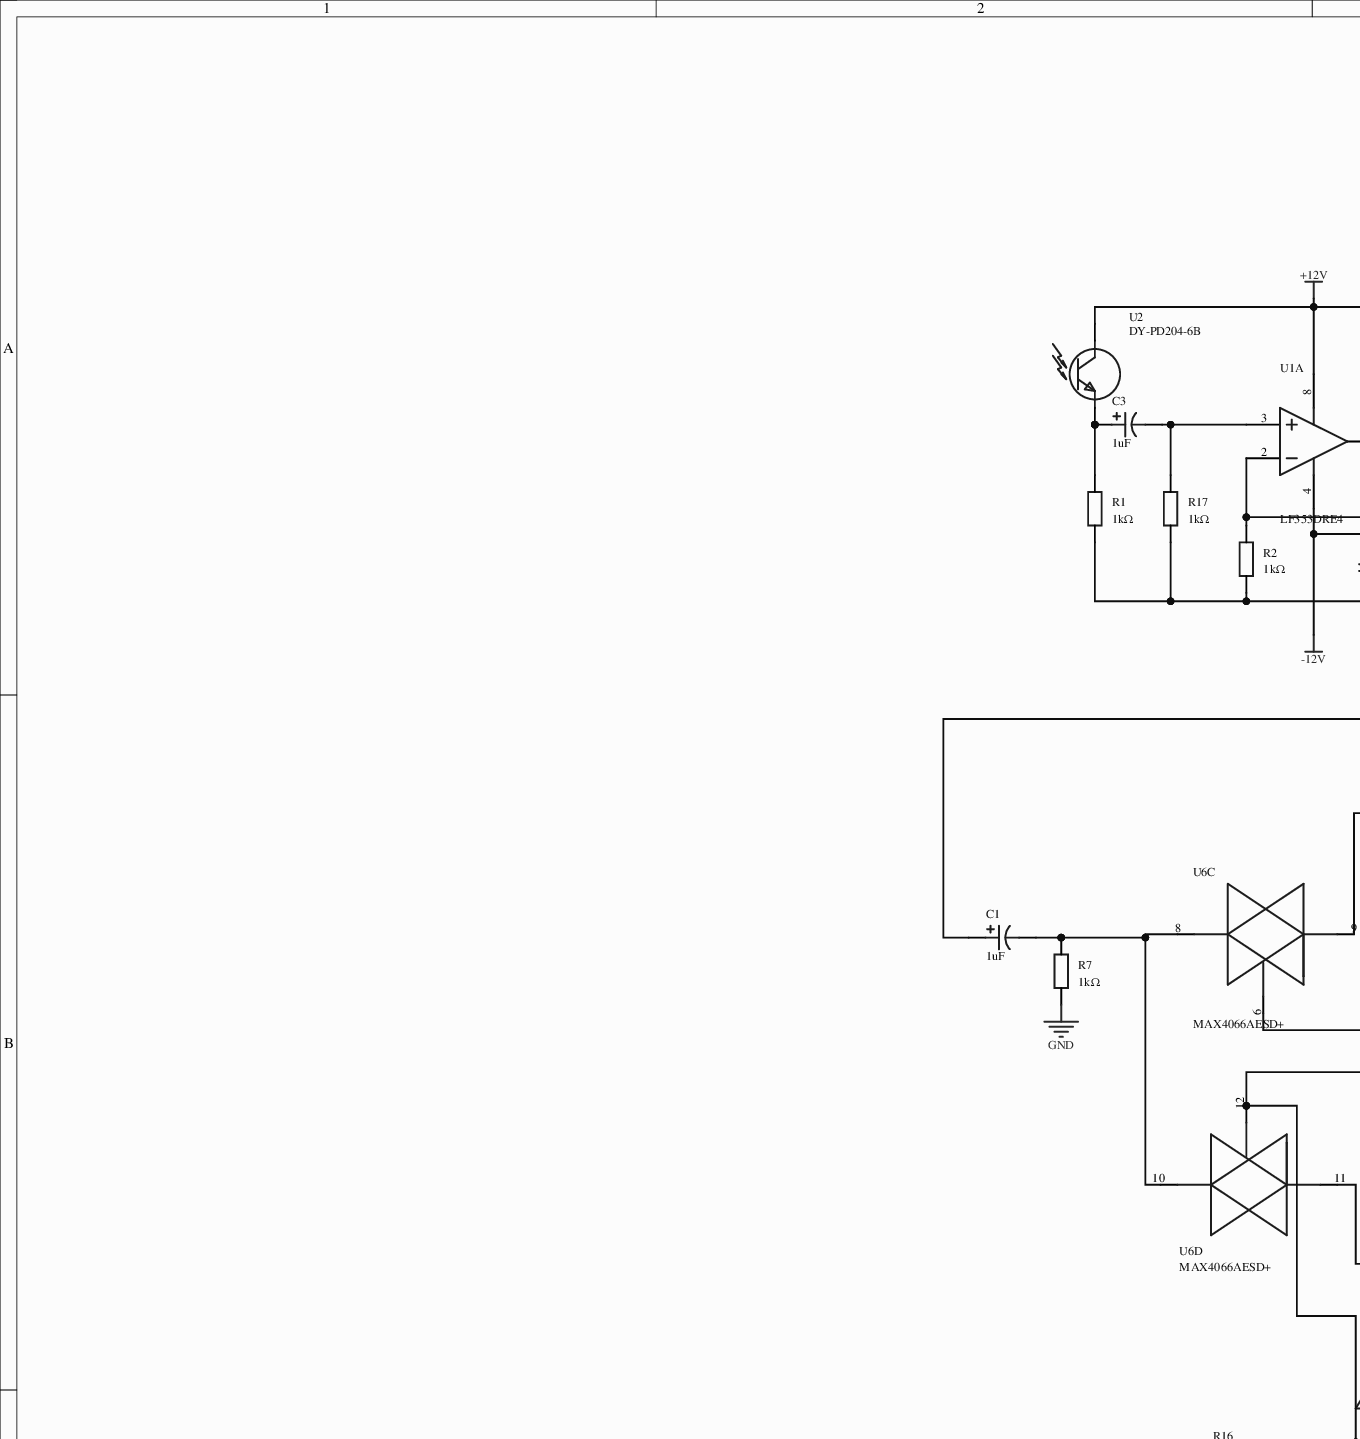
[diagram p0: MISC51811-3.schdoc, top left]
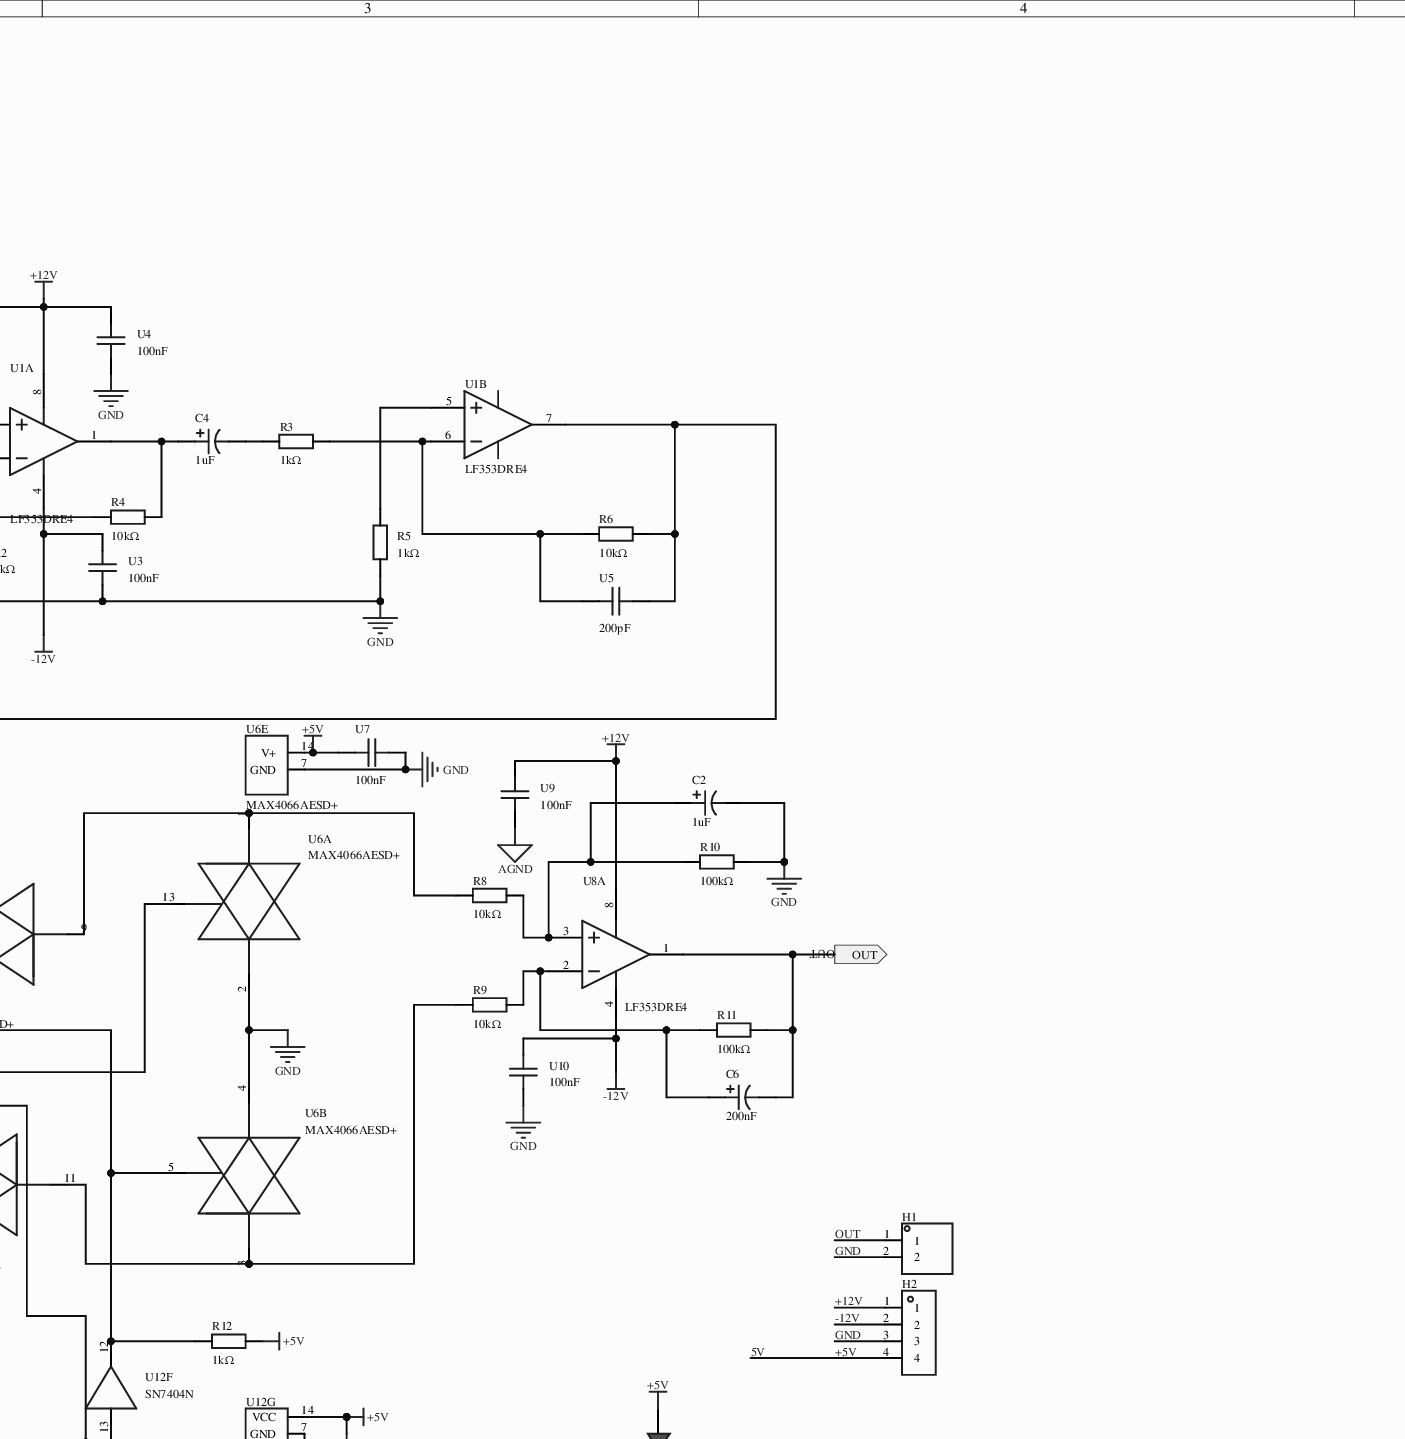
[diagram p1: MISC51811-3.schdoc, top middle]
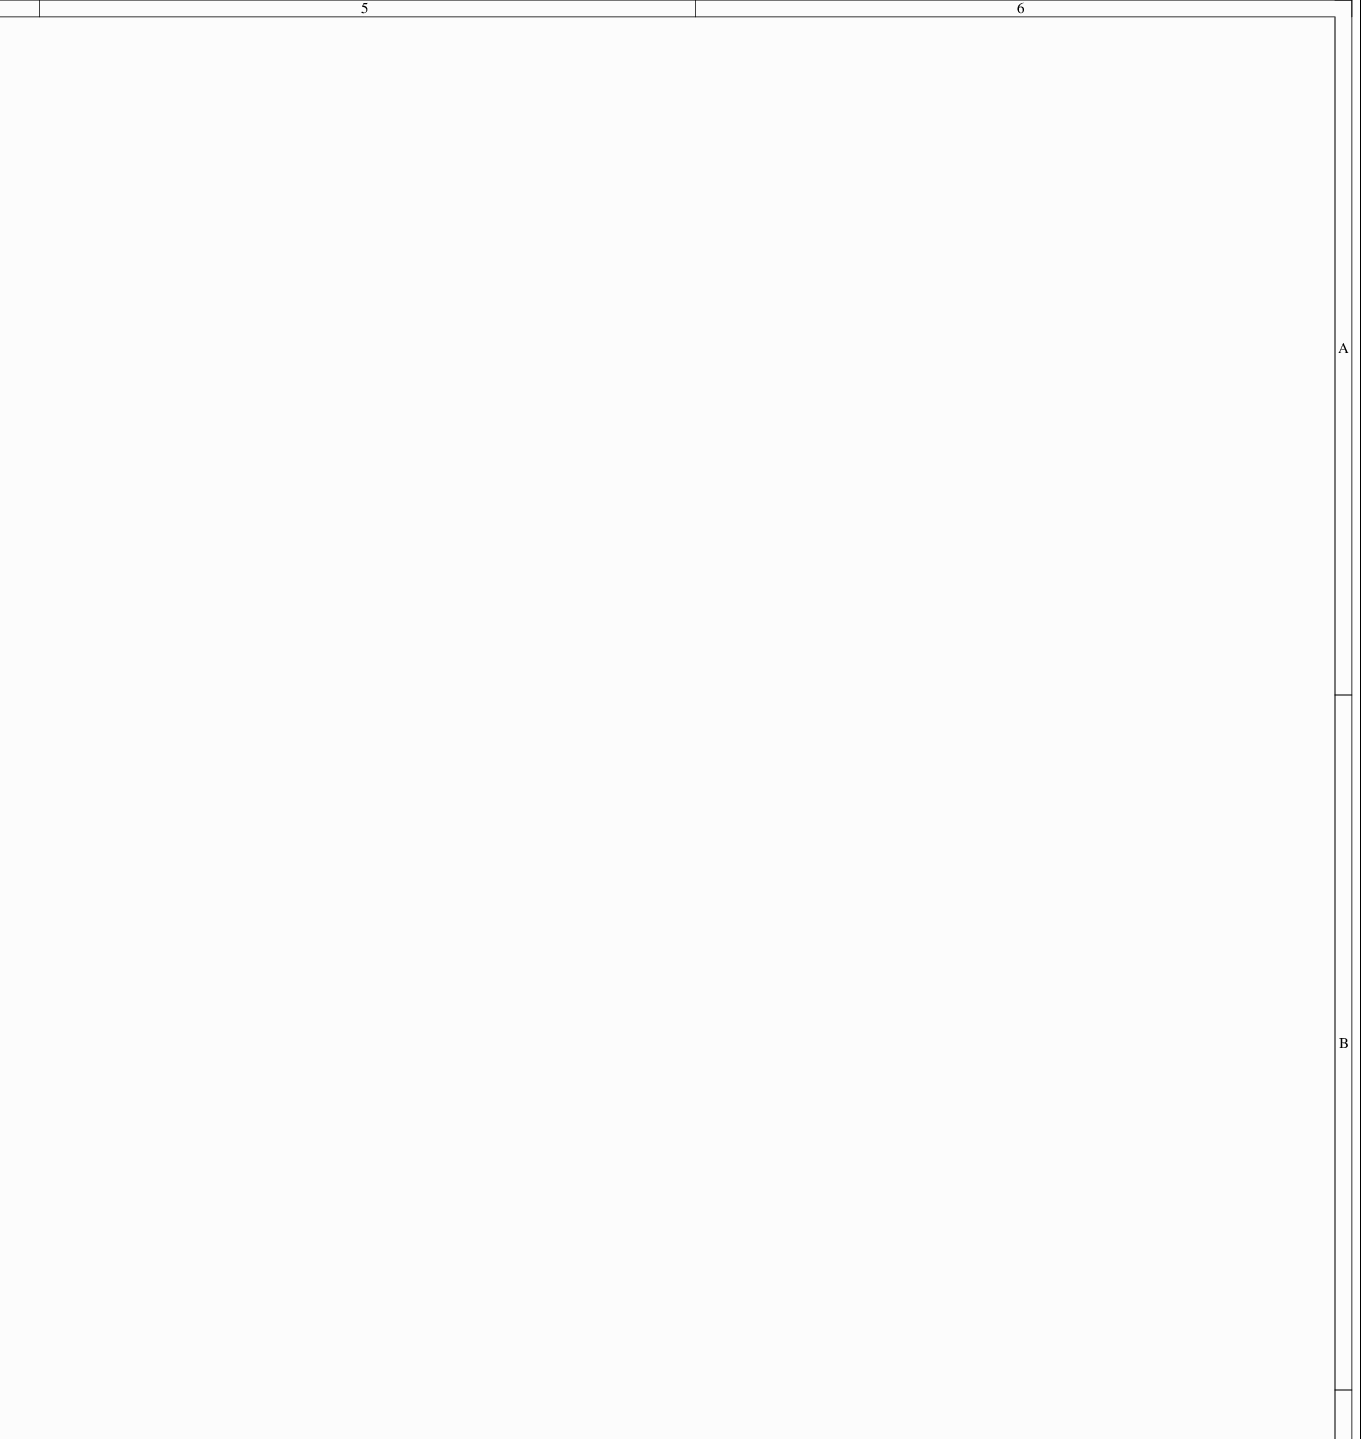
[diagram p2: MISC51811-3.schdoc, top right]
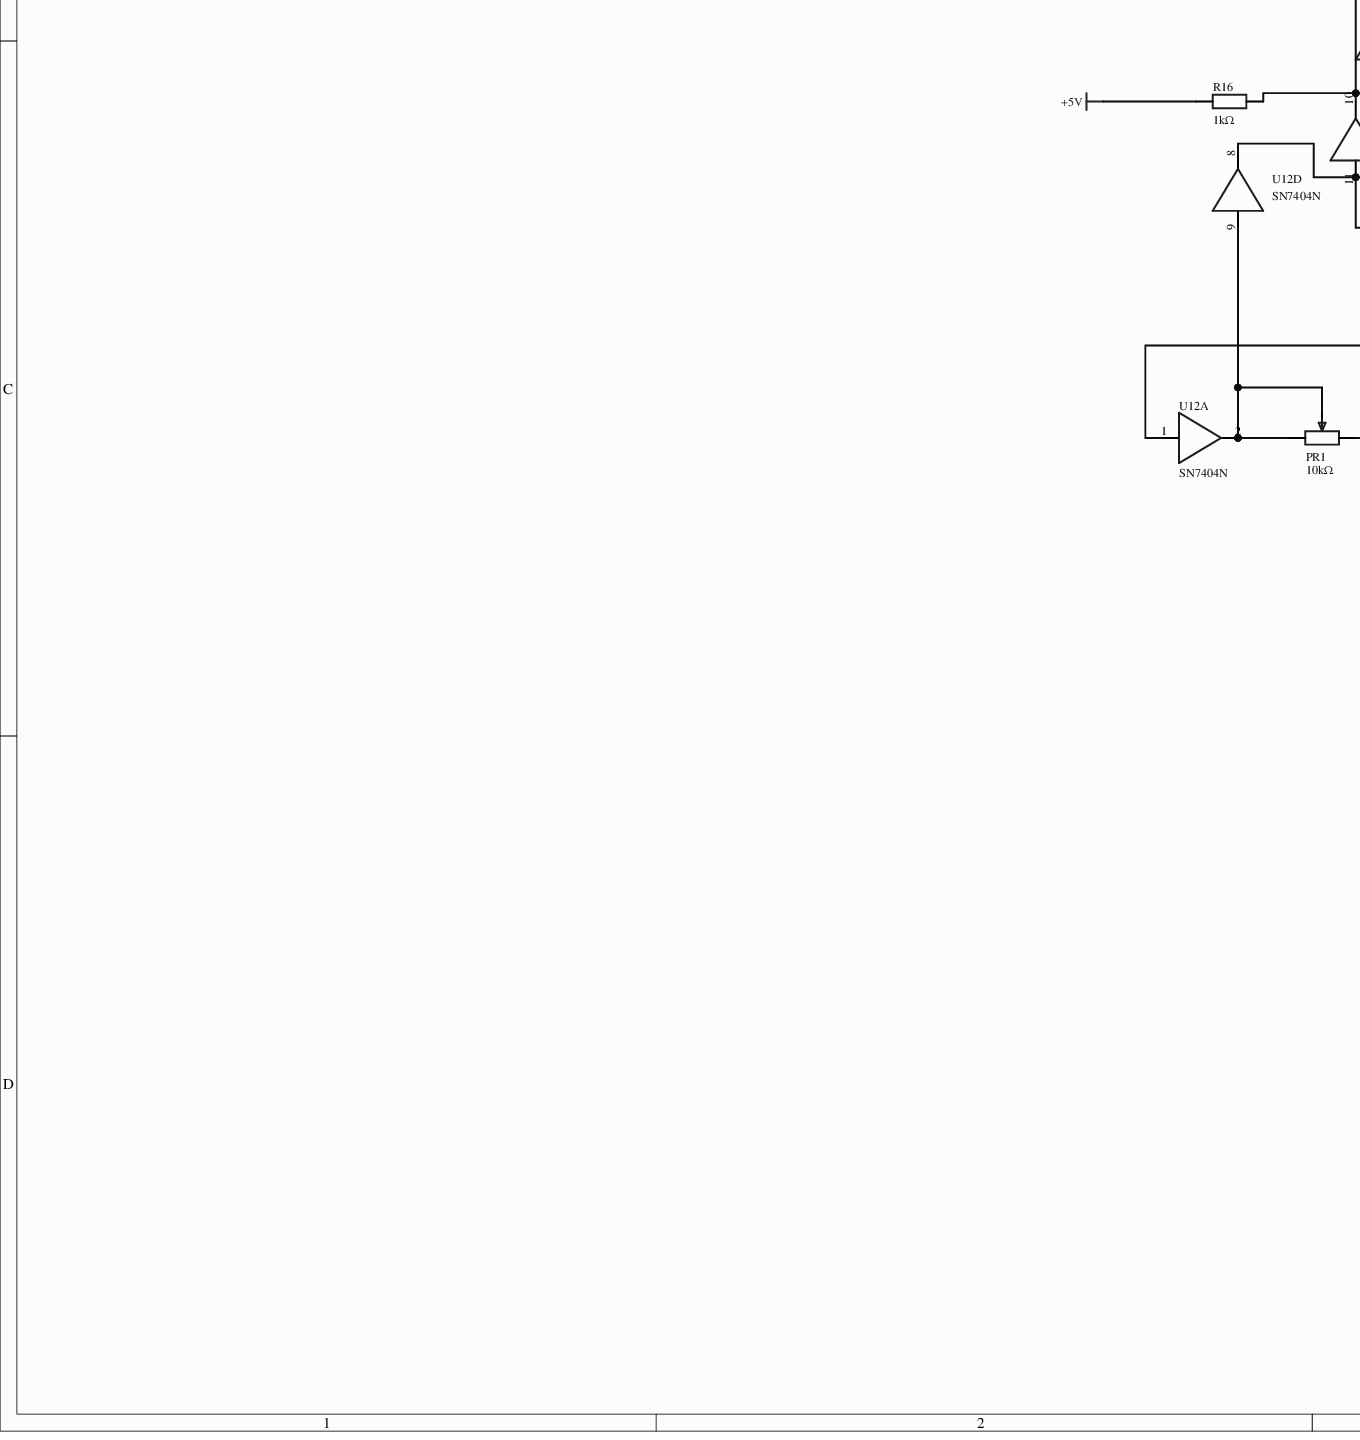
[diagram p3: MISC51811-3.schdoc, bottom left]
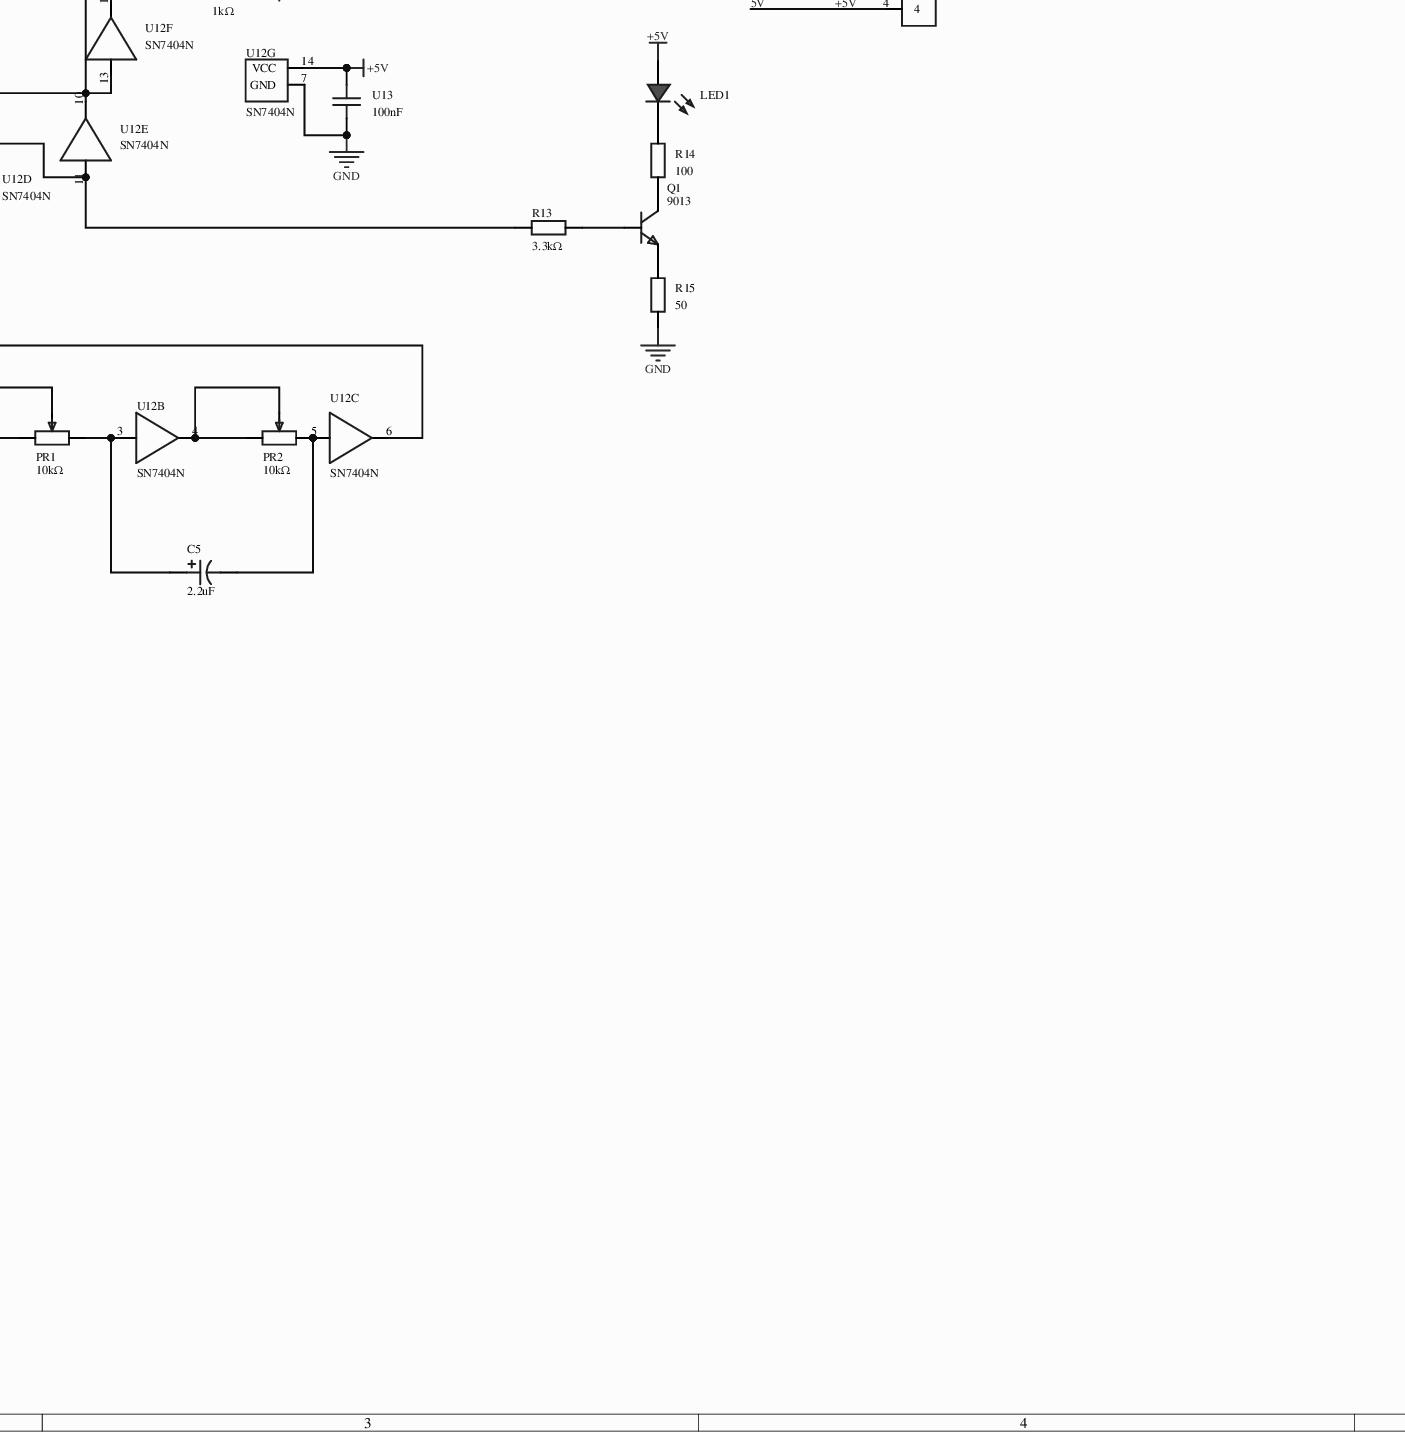
[diagram p4: MISC51811-3.schdoc, bottom middle]
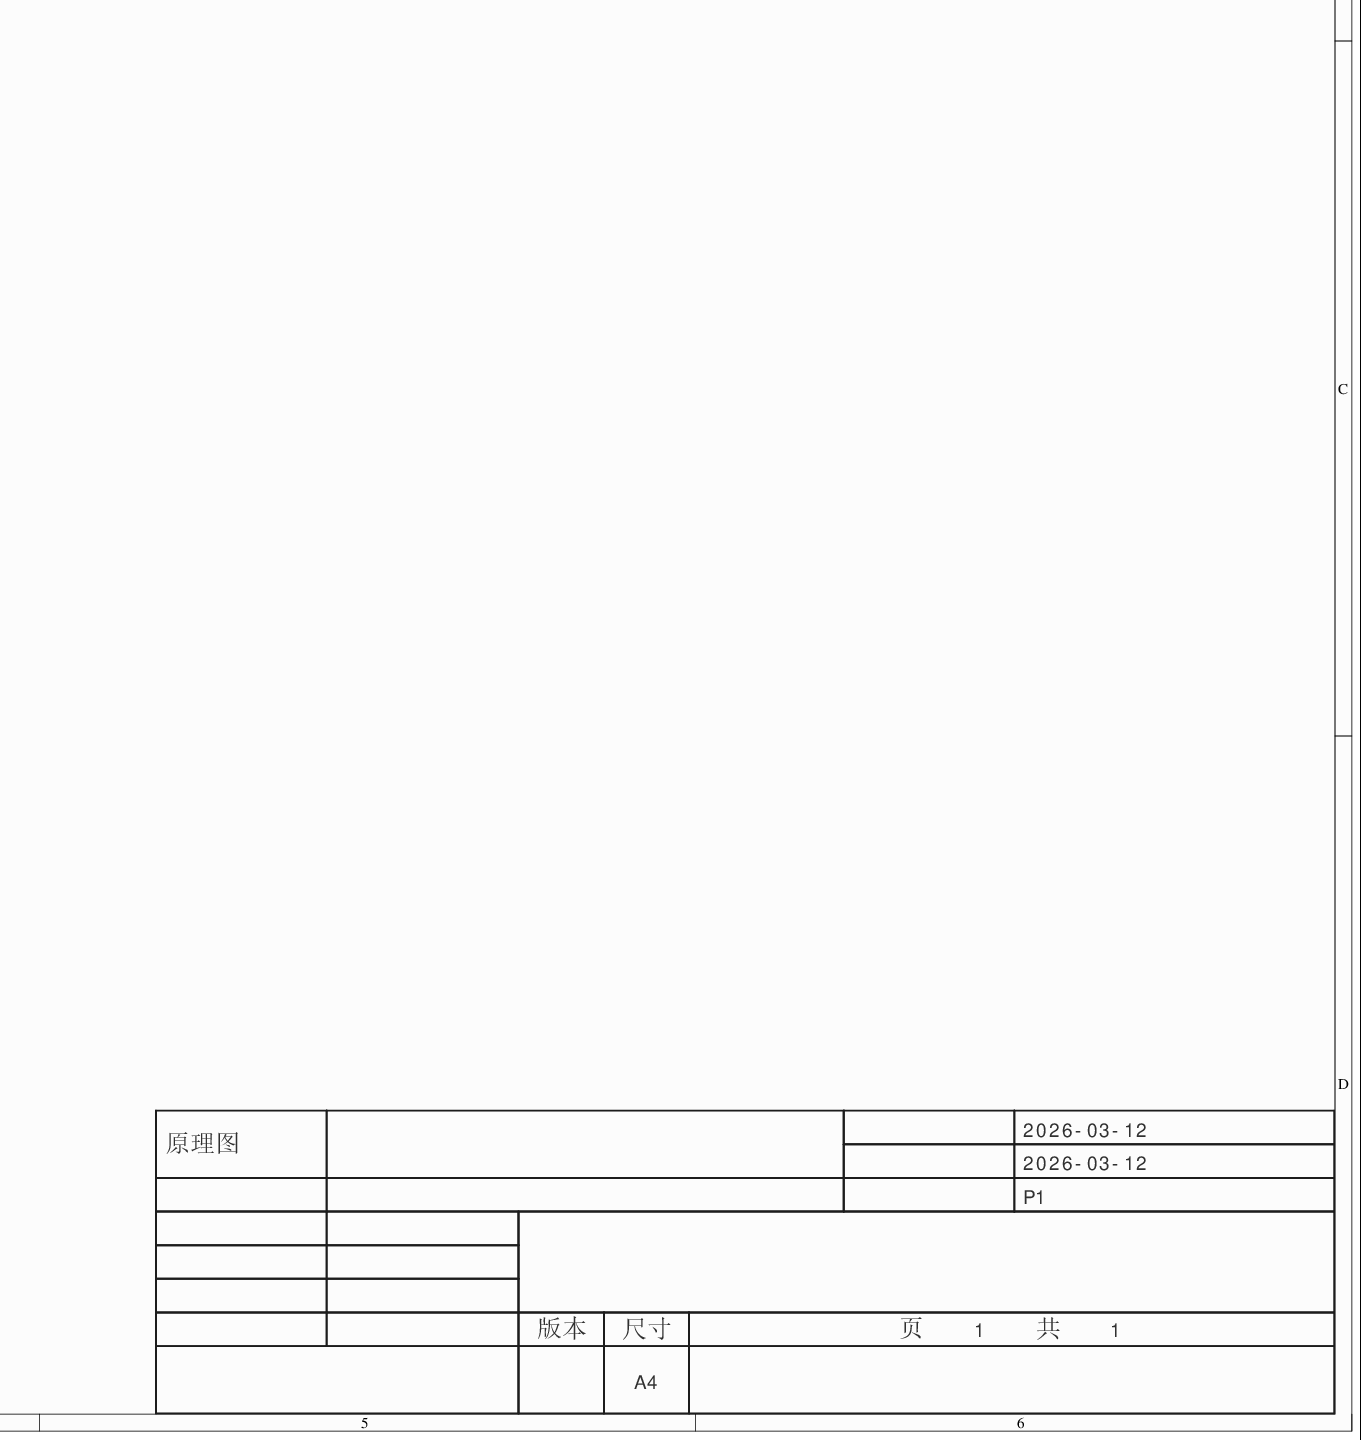
[diagram p5: MISC51811-3.schdoc, bottom right]
# Altium project MISC51811-2.PrjPcb
1 sheet, 41 parts. Net scope: flat (ports and power ports of the same name join across sheets).
Board file: MISC51811.pcbdoc

## Sheet MISC51811-3.schdoc
size 594 x 419 mm; Version: V1.0; @Project Name: MISC51811; @Update Date: 2026-03-12; @Create Date: 2026-03-12; @Board Name: MISC51811; @Create Time: 18:01:41; @Page Count: 1; @Page No: 1; @Schematic Name: MISC51811; @Update Time: 18:01:41; Size: A4

### Parts
C1  1uF  [CAP-TH_BD6.3-P2.50-D0.5-FD]
C2  1uF  [CAP-TH_BD6.3-P2.50-D0.5-FD]
C3  1uF  [CAP-TH_BD6.3-P2.50-D0.5-FD]
C4  1uF  [CAP-TH_BD6.3-P2.50-D0.5-FD]
C5  2.2uF  [CAP-TH_BD8.0-P3.50-D0.5-FD]
C6  200nF  [CAP-TH_BD6.3-P2.50-D0.5-FD]
H1  (no value)  [HDR-TH_2P-P2.54-V-M-1]
H2  (no value)  [HDR-TH_4P-P2.54-V-M]
LED1  (no value)  [LED_TH-3mm]
PR1  10kΩ  [R_3296]
PR2  10kΩ  [R_3296]
Q1  9013  [TO-92-3_L4.8-W3.7-P2.54-R]
R1  1kΩ  [Res_1/8W]
R2  1kΩ  [Res_1/8W]
R3  1kΩ  [Res_1/8W]
R4  10kΩ  [Res_1/8W]
R5  1kΩ  [Res_1/8W]
R6  10kΩ  [Res_1/8W]
R7  1kΩ  [Res_1/8W]
R8  10kΩ  [Res_1/8W]
R9  10kΩ  [Res_1/8W]
R10  100kΩ  [Res_1/8W]
R11  100kΩ  [Res_1/8W]
R12  1kΩ  [Res_1/8W]
R13  3.3kΩ  [Res_1/8W]
R14  100  [Res_1/8W]
R15  50  [Res_1/8W]
R16  1kΩ  [Res_1/8W]
R17  1kΩ  [Res_1/8W]
U1  LF353DRE4  [SOIC-8_L5.0-W4.0-P1.27-LS6.1-BL]  (parts A,B of 2)
U2  DY-PD204-6B  [LED-TH_BD3.0-P2.54-FD]
U3  100nF  [CAP-TH_L5.0-W2.5-P5.00-D1.0]
U4  100nF  [CAP-TH_L5.0-W2.5-P5.00-D1.0]
U5  200pF  [CAP-TH_L4.9-W3.7-P5.08-D0.5]
U6  MAX4066AESD+  [SOIC-14_L8.7-W3.9-P1.27-LS6.0-BL]  (parts A,B,C,D,E of 5)
U7  100nF  [CAP-TH_L5.0-W2.5-P5.00-D1.0]
U8  LF353DRE4  [SOIC-8_L5.0-W4.0-P1.27-LS6.1-BL]  (part A of 2)
U9  100nF  [CAP-TH_L5.0-W2.5-P5.00-D1.0]
U10  100nF  [CAP-TH_L5.0-W2.5-P5.00-D1.0]
U12  SN7404N  [PDIP-14_L19.3-W6.4-P2.54-LS7.9-BL-1]  (parts A,B,C,D,E,F,G of 8)
U13  100nF  [CAP-TH_L5.0-W2.5-P5.00-D1.0]

### Ports
OUT (out)

### Nets
+5V: H2.4 LED1.1(C) R12.1 R16.1 U6.14(V+) U7.1 U12.14(VCC) U13.2  [also labelled 5V]
+12V: H2.1 U1.8(VCC+) U2.2(C) U4.1 U8.8(VCC+) U9.2
-12V: H2.2 U1.4(VCC-) U3.1 U8.4(VCC-) U10.2
AGND: U9.1
GND: C2.2 H1.2 H2.3 R1.1 R2.1 R5.2 R7.1 R10.2 R15.1 R17.1 U3.2 U4.2 U6.2(COM1) U6.4(COM1) U6.7(GND) U7.2 U10.1 U12.7(GND) U13.1
OUT: C6.2 H1.1 R11.2 U8.1(1OUT) ; port OUT
NetC1_1: C1.1 R6.2 U1.7(2OUT) U5.2
NetC1_2: C1.2 R7.2 U6.8(COM1) U6.10(COM1)
NetC2_1: C2.1 R8.2 R10.1 U8.3(1IN-)
NetC3_1: C3.1 R1.2 U2.1(E)
NetC3_2: C3.2 R17.2 U1.3(1IN-)
NetC4_1: C4.1 R4.2 U1.1(1OUT)
NetC4_2: C4.2 R3.2
NetC5_1: C5.1 PR1.1 U12.3(1Y)
NetC5_2: C5.2 PR2.1 U12.5(1Y)
NetC6_1: C6.1 R9.2 R11.1 U8.2(1IN+)
NetLED1_2: LED1.2(A) R14.2
NetPR1_2: PR1.2 PR1.3 U12.2(1A) U12.9(1Y)
NetPR2_2: PR2.2 PR2.3 U12.4(1A)
NetQ1_1: Q1.1(C) R14.1
NetQ1_2: Q1.2(B) R13.2
NetQ1_3: Q1.3(E) R15.2
NetR2_2: R2.2 R4.1 U1.2(1IN+)
NetR3_1: R3.1 R6.1 U1.6(2IN-) U5.1
NetR5_1: R5.1 U1.5(2IN+)
NetR8_1: R8.1 U6.1(NO1) U6.9(NO1)
NetR9_1: R9.1 U6.3(NO1) U6.11(NO1)
NetR12_2: R12.2 U6.5(IN1) U6.6(IN1) U12.12(1A)
NetR13_1: R13.1 U12.8(1A) U12.11(1Y)
NetR16_2: R16.2 U6.12(IN1) U6.13(IN1) U12.10(1A) U12.13(1Y)
NetU12_1: U12.1(1Y) U12.6(1A)

### Notes on the sheet
- 2026-03-12
- 原理图
- P1
- 版本
- 尺寸
- A4
- 页    1    共    1

### Library data of the parts
C1-C4 = 1uF450V6.3x12KM: 容值:1uF;精度:±20%;额定电压:450V;纹波电流:545mA@120Hz;等效串联电阻(ESR):11Ω;; Manufacturer: Econd(米朗电子); AddInBom: yes; ModelId: 983aa343eddc42b59ebb10541a88166e0819f05c4eef4c71ace90d822a990e87; ModelTransform: 247.99486,248.229,0,90,0,0,0,0,-196.85; Tolerance: ±20%; Voltage Rating: 450V; Equivalent Series Resistance(ESR): 11Ω; Pin Spacing: 2.5mm; Lifetime: 2000hrs@105℃; Symbol: 1UF450V6.3X12KM; Device: 1uF450V6.3x12KM; LCSC Part Name: 1uF ±20% 450V; SupplierPart: C49304904; ManufacturerPart: 1uF450V6.3x12KM; Supplier Footprint: 插件,D6.3xL12mm; JLCPCB Part Class: Extended Part; Datasheet: https://item.szlcsc.com/datasheet/1uF450V6.3x12KM/51766732.html; Supplier: LCSC; ConvertToPcb: yes; FootprintName: CAP-TH_BD6.3-P2.50-D0.5-FD; ModelName: CAP-TH_BD6.3-P2.50-D0.5-FD; Value: 1uF; Ripple Current: 545mA@120Hz; Diameter: 6.3mm; Height - Seated (Max): 12mm; Operating Temperature: -25℃~+105℃
C5 = 2.2uF450V8x12KM: 容值:2.2uF;精度:±20%;额定电压:450V;纹波电流:35mA@120HZ;等效串联电阻(ESR):11Ω;; Manufacturer: Econd(米朗电子); AddInBom: yes; ModelId: 627d55c9ca1c4b51a61bba7c83a7ae6f0819f05c4eef4c71ace90d822a990e87; ModelTransform: 314.96,315.3537,0,90,0,0,0,0,-196.85; Tolerance: ±20%; Voltage Rating: 450V; Equivalent Series Resistance(ESR): 11Ω; Pin Spacing: 3.5mm; Lifetime: 2000hrs@105℃; Symbol: 2.2UF450V8X12KM; Device: 2.2uF450V8x12KM; LCSC Part Name: 2.2uF ±20% 450V; SupplierPart: C49304892; ManufacturerPart: 2.2uF450V8x12KM; Supplier Footprint: 插件,D8xL12mm; JLCPCB Part Class: Extended Part; Datasheet: https://item.szlcsc.com/datasheet/2.2uF450V8x12KM/51766720.html; Supplier: LCSC; ConvertToPcb: yes; FootprintName: CAP-TH_BD8.0-P3.50-D0.5-FD; ModelName: CAP-TH_BD8.0-P3.50-D0.5-FD; Value: 2.2uF; Ripple Current: 35mA@120HZ; Diameter: 8mm; Height - Seated (Max): 12mm; Operating Temperature: -25℃~+105℃
C6 = 1uF450V6.3x12KM: 容值:1uF;精度:±20%;额定电压:450V;纹波电流:545mA@120Hz;等效串联电阻(ESR):11Ω;; Manufacturer: Econd(米朗电子); 3D Model: 983aa343eddc42b59ebb10541a88166e0819f05c4eef4c71ace90d822a990e87; 3D Model Transform: 247.99486,248.229,0,90,0,0,0,0,-196.85; Tolerance: ±20%; Voltage Rating: 450V; Equivalent Series Resistance(ESR): 11Ω; Pin Spacing: 2.5mm; Lifetime: 2000hrs@105℃; AddInBom: yes; Symbol: 1UF450V6.3X12KM; Device: 1uF450V6.3x12KM; LCSC Part Name: 1uF ±20% 450V; Manufacturer Part: 1uF450V6.3x12KM; Supplier Footprint: 插件,D6.3xL12mm; JLCPCB Part Class: Extended Part; Datasheet: https://item.szlcsc.com/datasheet/1uF450V6.3x12KM/51766732.html; Supplier: LCSC; Value: 200nF; Ripple Current: 545mA@120Hz; Diameter: 6.3mm; Height - Seated (Max): 12mm; Operating Temperature: -25℃~+105℃; ConvertToPcb: yes; FootprintName: CAP-TH_BD6.3-P2.50-D0.5-FD; ModelName: CAP-TH_BD6.3-P2.50-D0.5-FD
H1 = HDR-M_2.54_1x2P: Symbol: 210S-1*2P L=11.6MMGold-plated black; ConvertToPcb: yes; ModelId: 79b2e9f2d70a4d68a1b7098f27c6d4c50819f05c4eef4c71ace90d822a990e87; ModelName: HDR-M-2.54_1x2; ModelTransform: 200,100,0,0,0,0,0,0,-118.11; Device: HDR-M_2.54_1x2P; AddInBom: yes; SupplierPart: C124375; Supplier Footprint: 插件; FootprintName: HDR-TH_2P-P2.54-V-M-1
H2 = HDR-M_2.54_1x4P: Symbol: PZ254V-11-04P; ConvertToPcb: yes; ModelId: 112f4d05e8d64e99ab9a333894bea4f90819f05c4eef4c71ace90d822a990e87; ModelName: HDR-TH_4P-P2.54-M-LI-1X4P; ModelTransform: 399.999,104.7242,0,0,0,0,0,0,-118.11; Device: HDR-M_2.54_1x4P; AddInBom: yes; SupplierPart: C492403; Supplier Footprint: 插件; FootprintName: HDR-TH_4P-P2.54-V-M
LED1 = LED_TH-R_3mm: ConvertToPcb: yes; ModelId: a497c992633541038a38947cdc58012f0819f05c4eef4c71ace90d822a990e87; ModelName: LED-TH-3mm_R; ModelTransform: 141.274,153.327,0,0,0,0,-5.984,0,-137.795; Symbol: LED_TH-R; Device: LED_TH-R_3mm; AddInBom: yes; FootprintName: LED_TH-3mm; Supplier Footprint: 插件
PR1 PR2 = R_3296: ConvertToPcb: yes; ModelId: b182808559bb43bda9e7de64b64134cb0819f05c4eef4c71ace90d822a990e87; ModelName: 3296W; ModelTransform: 373.98,188.96,590.49,180,0,0,0,0,-140; Symbol: R_3296; Device: R_3296; AddInBom: yes; Supplier Footprint: 直插; FootprintName: R_3296; Value: 10kΩ
Q1 = 9013: 晶体管类型:NPN;集电极电流(Ic):500mA;集射极击穿电压(Vceo):20V;耗散功率(Pd):625mW;直流电流增益(hFE):276@50mA,1.0V;; Manufacturer: BLUE ROCKET(蓝箭); AddInBom: yes; ModelId: 0fb83455cf6d479b95862acdd73b6eef0819f05c4eef4c71ace90d822a990e87; ModelName: TO-92-3_L4.8-W3.7-H7.7-P2.54-R; ModelTransform: 218.897,161.417,0,180,0,0,0,13.78,-433.071; type: NPN; Current - Collector(Ic): 500mA; Collector - Emitter Voltage VCEO: 20V; Pd - Power Dissipation: 625mW; Current - Collector Cutoff: 100nA; Vce Saturation(VCE(sat)): 600mV@500mA,50mA; Emitter-Base Voltage(Vebo): 5V; Number: 1个NPN; Symbol: 9013; Device: 9013; LCSC Part Name: TO-92塑封封装NPN半导体三极管 NPN 电流:500mA 电压:20V; SupplierPart: C3037603; ManufacturerPart: 9013; Supplier Footprint: TO-92-2.54mm; JLCPCB Part Class: Extended Part; Datasheet: https://item.szlcsc.com/datasheet/9013/3589217.html; Supplier: LCSC; ConvertToPcb: yes; FootprintName: TO-92-3_L4.8-W3.7-P2.54-R; DC Current Gain: 276@50mA,1.0V
R1-R16 = Res_AXIAL-1/8W: Symbol: 电阻; ConvertToPcb: yes; ModelId: b2b5ae7ae4c642178fe0039925c86a3f0819f05c4eef4c71ace90d822a990e87; ModelName: RES-TH_BD1.8-L3.2-P7.20-D0.4; ModelTransform: 282.86,66.88,253.09,0,0,0,0,0,-191; Device: Res_AXIAL-1/8W; AddInBom: yes; Supplier Footprint: 轴向引线; FootprintName: Res_1/8W
  R1-R3 R5 R7 R12 R16: Value: 1kΩ
  R4 R6 R8 R9: Value: 10kΩ
  R10 R11: Value: 100kΩ
  R13: Value: 3.3kΩ
  R14: Value: 100
  R15: Value: 50
R17 = Res_AXIAL-1/8W: Symbol: 电阻; 3D Model: b2b5ae7ae4c642178fe0039925c86a3f0819f05c4eef4c71ace90d822a990e87; 3D Model Transform: 282.86,66.88,253.09,0,0,0,0,0,-191; ConvertToPcb: yes; ModelName: RES-TH_BD1.8-L3.2-P7.20-D0.4; Device: Res_AXIAL-1/8W; Value: 1kΩ; Supplier Footprint: 轴向引线; AddInBom: yes; FootprintName: Res_1/8W
U1 U8 = LF353DRE4: 增益带宽积(GBP):3MHz;输入偏置电流(Ib):50pA;输入失调电压(Vos):5mV;压摆率(SR):13V/us;; Manufacturer: TI(德州仪器); Relevance: []; AddInBom: yes; ModelId: e95f26ea62414da0907e5731acbf3c9b0819f05c4eef4c71ace90d822a990e87; ModelTransform: 192.913,236.22,0,0,0,0,0,0,0; Gain Bandwidth Product(GBP): 3MHz; Current - Input Bias(Ib): 50pA; Voltage - Input Offset(Vos): 5mV; Slew Rate(SR): 13V/us; Symbol: LF353DRE4; Device: LF353DRE4; LCSC Part Name: LF353DRE4; SupplierPart: C2057895; ManufacturerPart: LF353DRE4; Supplier Footprint: SOIC-8; JLCPCB Part Class: Extended Part; Datasheet: https://www.ti.com/cn/lit/gpn/lf353; Supplier: LCSC; ConvertToPcb: yes; FootprintName: SOIC-8_L5.0-W4.0-P1.27-LS6.1-BL; ModelName: SOIC-8_L5.0-W4.0-P1.27-LS6.1-BL; Operating Temperature: 0℃~+70℃
U2 = DY-PD204-6B: DY-PD204-6B 是一种 NPN 型高速度和高敏感的光敏二极管。; Manufacturer: TONYU(东裕); AddInBom: yes; ModelId: a497c992633541038a38947cdc58012f0819f05c4eef4c71ace90d822a990e87; ModelName: LED-TH-3mm_R; ModelTransform: 141.274,153.327,0,0,0,0,-5.984,0,-137.795; Measurement Type: 光强; Symbol: DY-PD204-6B; Device: DY-PD204-6B; LCSC Part Name: 光敏二极管; SupplierPart: C841507; ManufacturerPart: DY-PD204-6B; Supplier Footprint: 插件,D=3mm; JLCPCB Part Class: Extended Part; Datasheet: https://item.szlcsc.com/datasheet/DY-PD204-6B/899044.html; Supplier: LCSC; ConvertToPcb: yes; FootprintName: LED-TH_BD3.0-P2.54-FD; Operating Temperature: -40℃~+85℃; Width: 2.54mm
U3 U4 U7 U9 U10 U13 = 100nF: Symbol: 100NF_C9900015256; AddInBom: yes; ModelId: 08e3d7481fc7486bb1b263873f51e1e10819f05c4eef4c71ace90d822a990e87; ModelName: CAP-TH_BD5.0-W2.5-P5.08; ModelTransform: 224.652,98.425,0,0,0,0,-0.005,0,-137.795; Device: 100nF; LCSC Part Name: 100nF; SupplierPart: C9900015256; ManufacturerPart: 100nF; Supplier Footprint: CAP-TH_L5.0-W2.5-P5.00-D1.0; JLCPCB Part Class: Extended Part; Supplier: LCSC; ConvertToPcb: yes; FootprintName: CAP-TH_L5.0-W2.5-P5.00-D1.0
U5 = CC4-0805-CG-100V-200PF-J: 容值:200pF;精度:±5%;额定电压:100V;温度系数:-;; Manufacturer: TORCH(火炬); AddInBom: yes; ModelId: d480a48107b54a3595d34e62c8baa7590819f05c4eef4c71ace90d822a990e87; ModelName: CAP-TH_L4.9-W3.7-H2.5-P5.08; ModelTransform: 215.7476,125.984,0,0,0,0,0,0,-137.795; Tolerance: ±5%; Voltage Rating: 100V; Symbol: CC4-0805-CG-100V-200PF-J; Device: CC4-0805-CG-100V-200PF-J; LCSC Part Name: 200pF ±5% 100V; SupplierPart: C400086; ManufacturerPart: CC4-0805-CG-100V-200PF-J; Supplier Footprint: 插件,P=5.08mm; JLCPCB Part Class: Extended Part; Datasheet: https://item.szlcsc.com/datasheet/CC4-0805-CG-100V-200PF-J/383459.html; Supplier: LCSC; ConvertToPcb: yes; FootprintName: CAP-TH_L4.9-W3.7-P5.08-D0.5; Value: 200pF; Temperature Coefficient: -
U6 = MAX4066AESD+: 开关电路:1:1;通道数:4;导通电阻(Ron):45Ω;; Manufacturer: ADI(亚德诺)/MAXIM(美信); Relevance: []; Add into BOM: yes; 3D Model: 8dbf5b715d42428c85558507ae5a252b0819f05c4eef4c71ace90d822a990e87; 3D Model Transform: 338.583,236.22,0,0,0,0,0,0.001,0; Switch Circuit: 1:1; Number of Channels: 4; Voltage - Supply: 2V~16V; Turn-on time: 150ns; Ron: 45Ω; Turn-off time: 75ns; Bandwidth: 100MHz; ModelName: SOIC-14_L8.6-W3.9-H1.8-LS6.0-P1.27; Symbol: MAX4066AESD+; Device: MAX4066AESD+; Convert to PCB: yes; LCSC Part Name: 低成本、低电压、四路、SPST、CMOS模拟开关; Supplier Part: C7458661; Manufacturer Part: MAX4066AESD+; Supplier Footprint: SOIC-14; JLCPCB Part Class: Extended Part; Datasheet: https://item.szlcsc.com/datasheet/MAX4066AESD%252B/8484762.html; Supplier: LCSC; Operating Temperature: -40℃~+85℃; FootprintName: SOIC-14_L8.7-W3.9-P1.27-LS6.0-BL
U12 = SN7404N: SN7404 6 通道、4.75V 至 5.25V 双极反相器; Manufacturer: TI(德州仪器); Add into BOM: yes; 3D Model: 850da569defe42bfb44bffbf615858220819f05c4eef4c71ace90d822a990e87; 3D Model Transform: 751.967,309.842,0,0,0,0,0,0,-118.11; Symbol: SN7404N; Device: SN7404N; Convert to PCB: yes; LCSC Part Name: 六独立反相器 - SN7404, SN74LS04, SN74S04; Supplier Part: C131919; Manufacturer Part: SN7404N; Supplier Footprint: PDIP-14; JLCPCB Part Class: Extended Part; Datasheet: https://www.ti.com/cn/lit/gpn/sn74ls04; Supplier: LCSC; FootprintName: PDIP-14_L19.3-W6.4-P2.54-LS7.9-BL-1; ModelName: PDIP-14_L19.3-W6.4-P2.54-LS7.9-BL-1